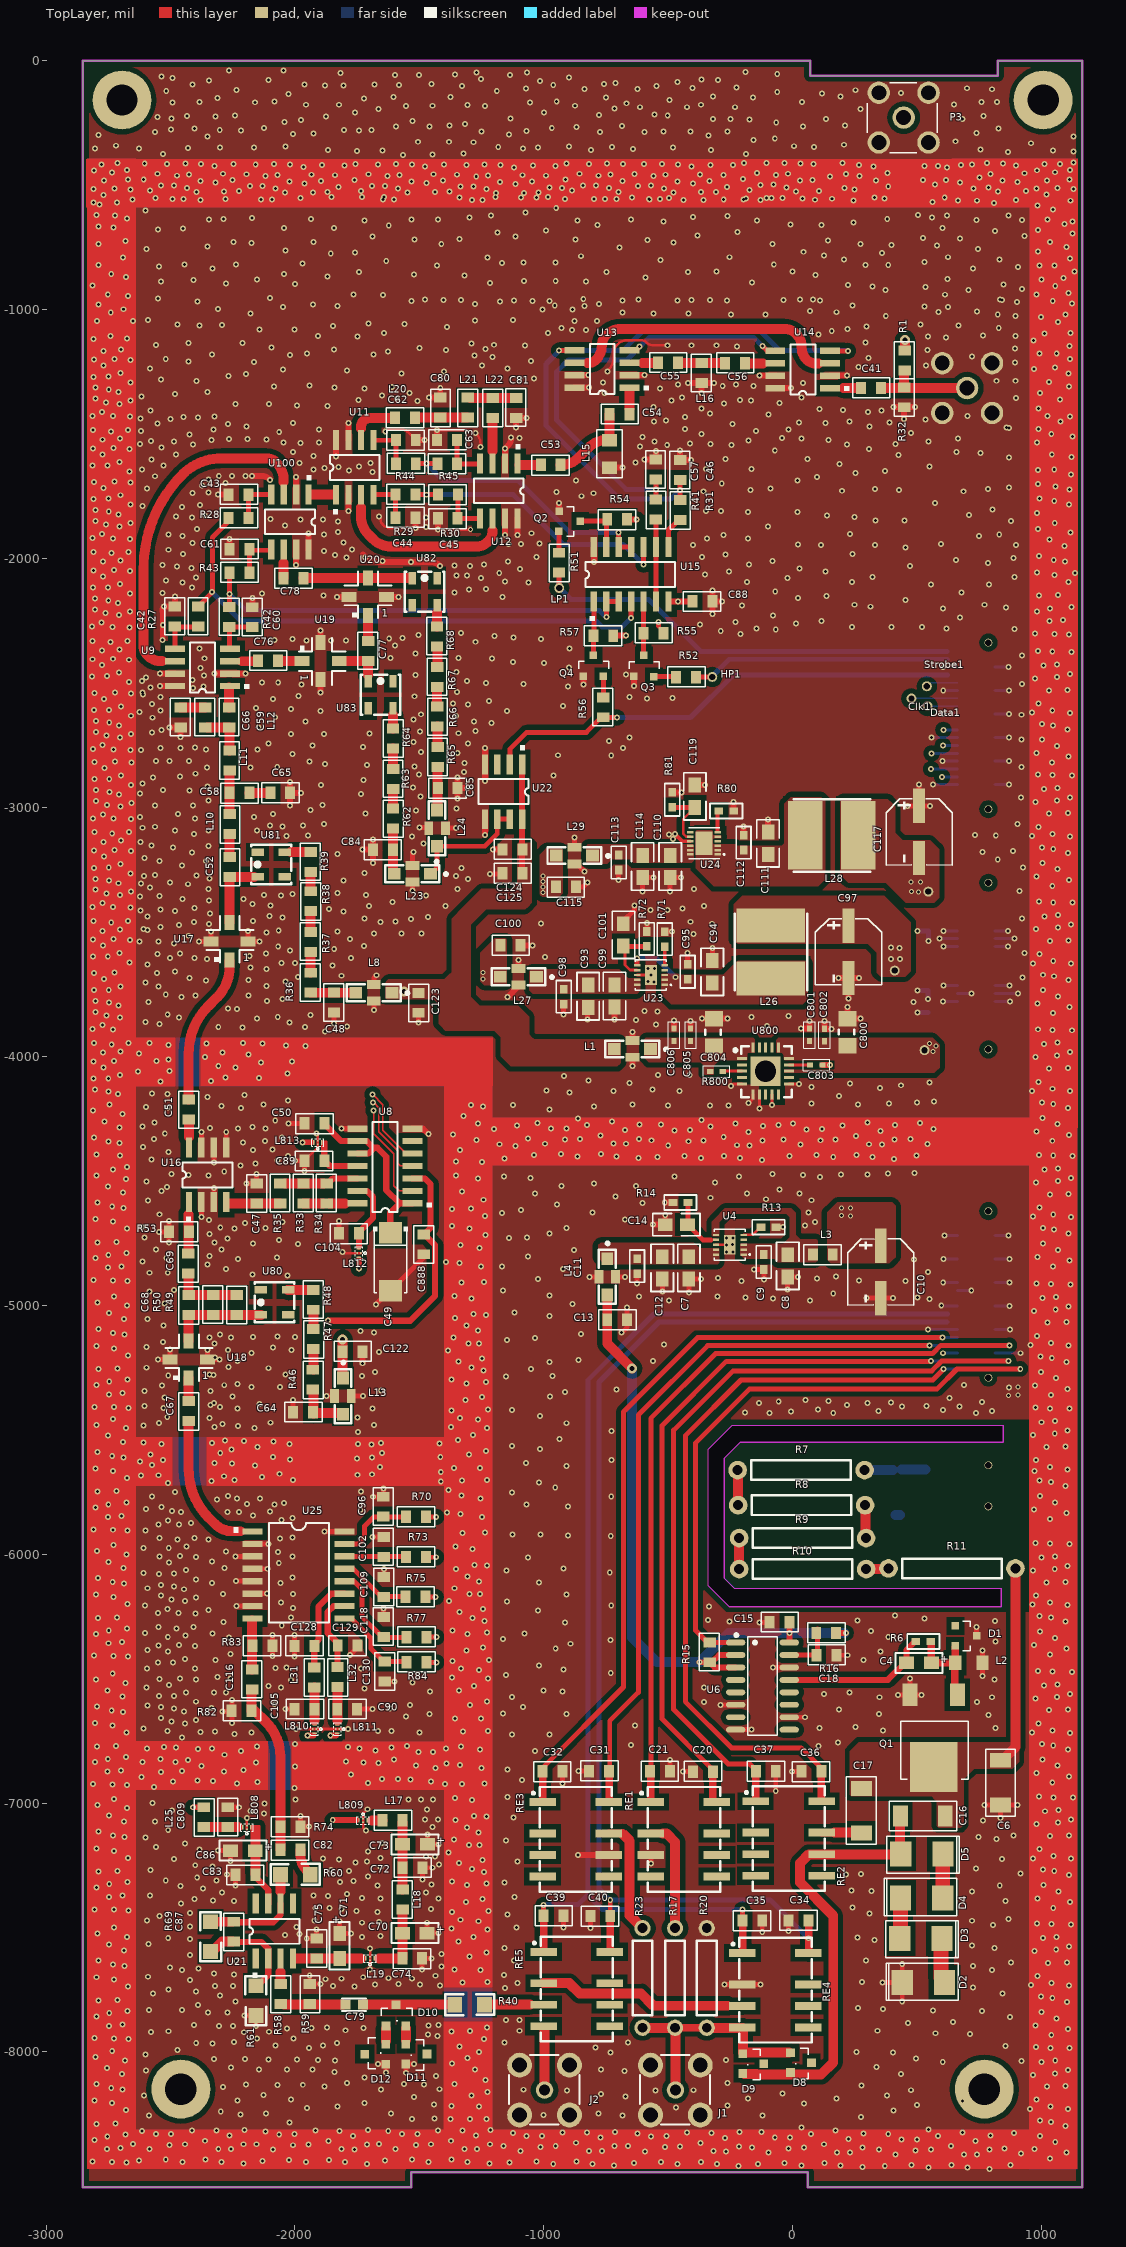
[diagram p0: TopLayer view]
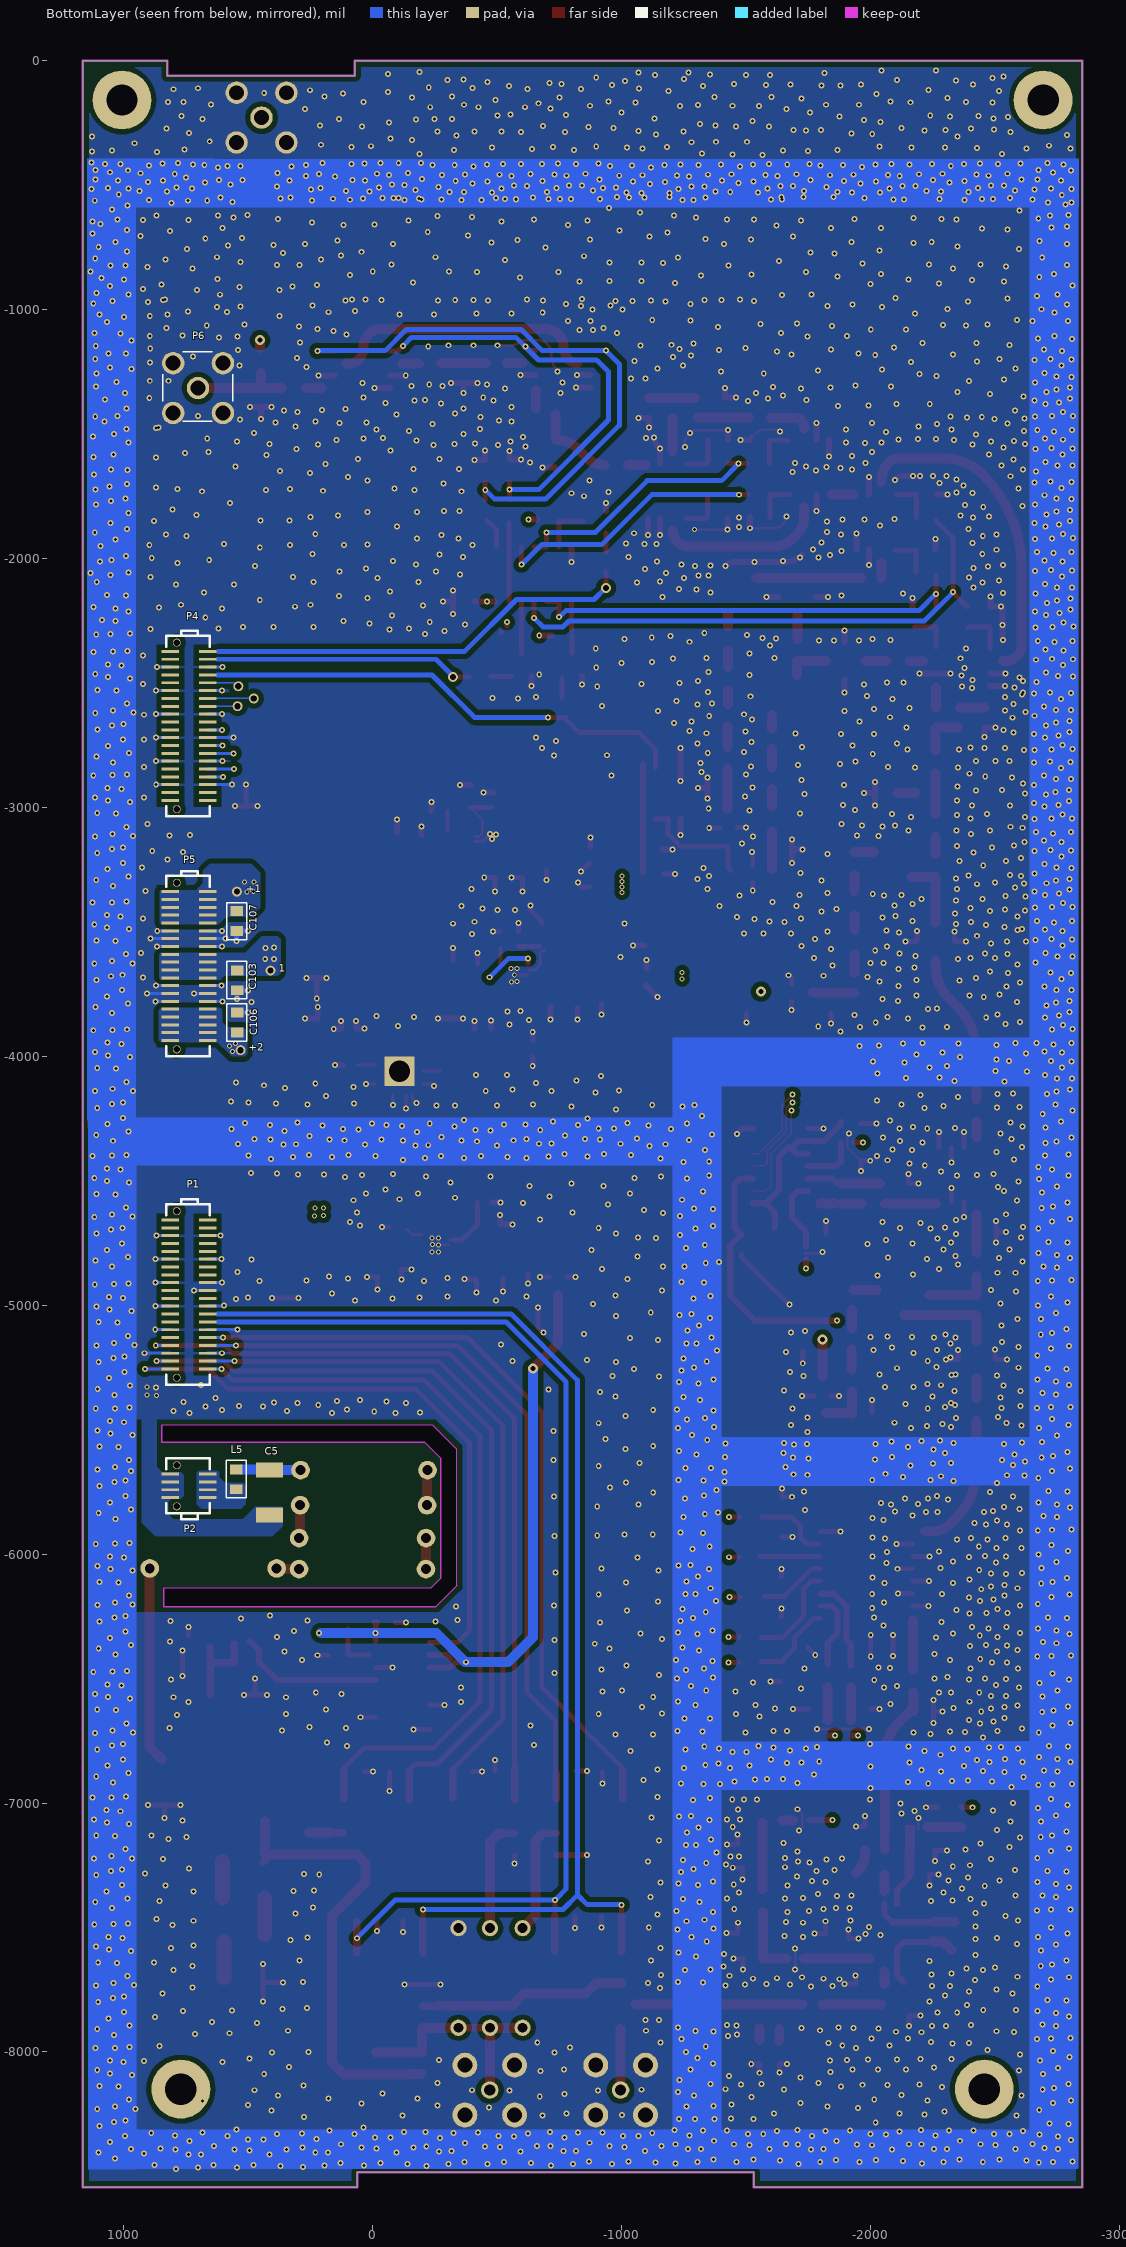
[diagram p1: BottomLayer view, seen from below]
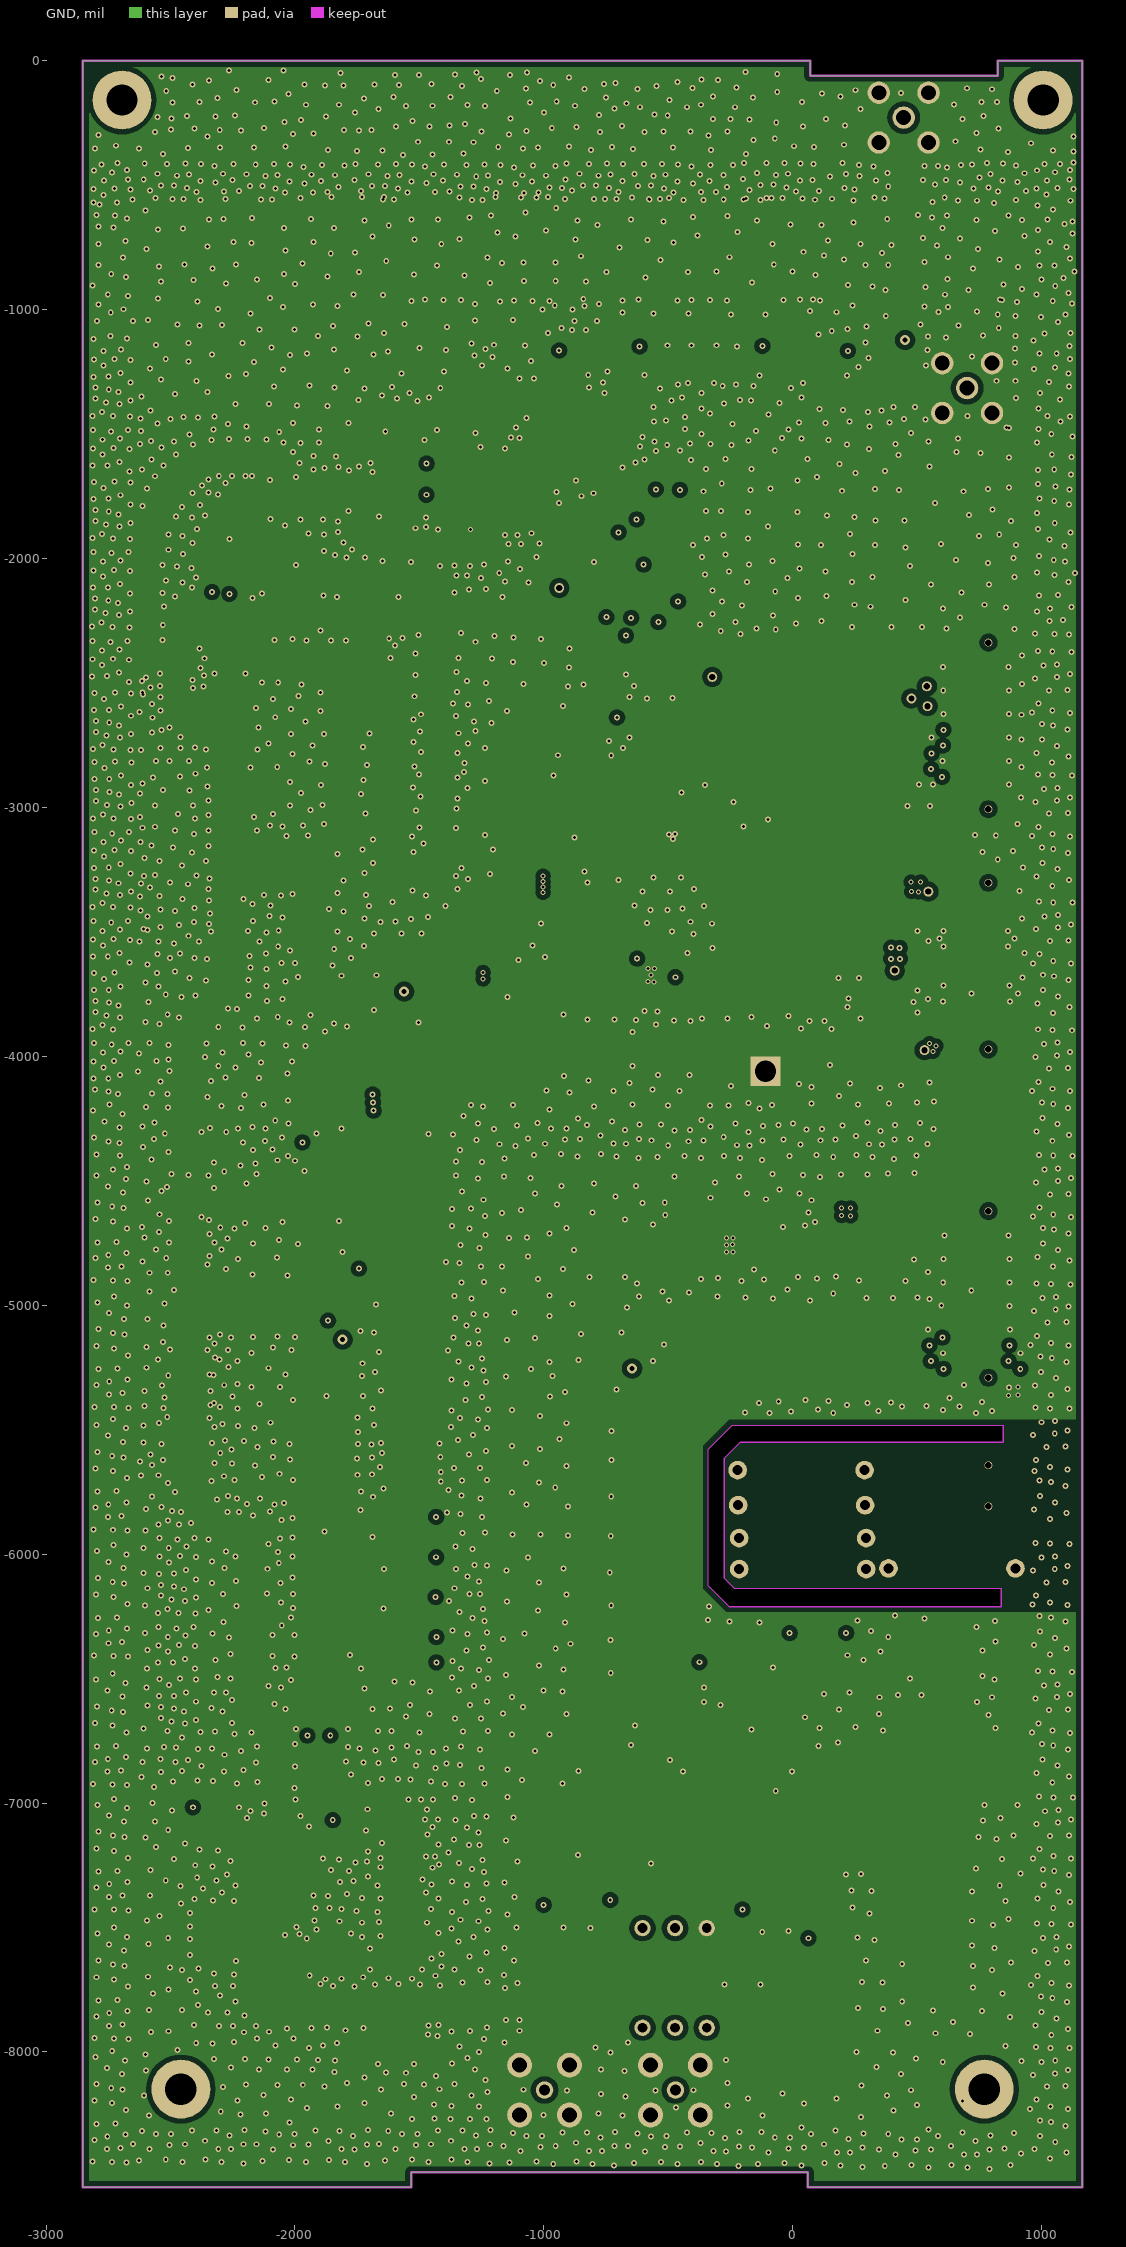
[diagram p2: GND]
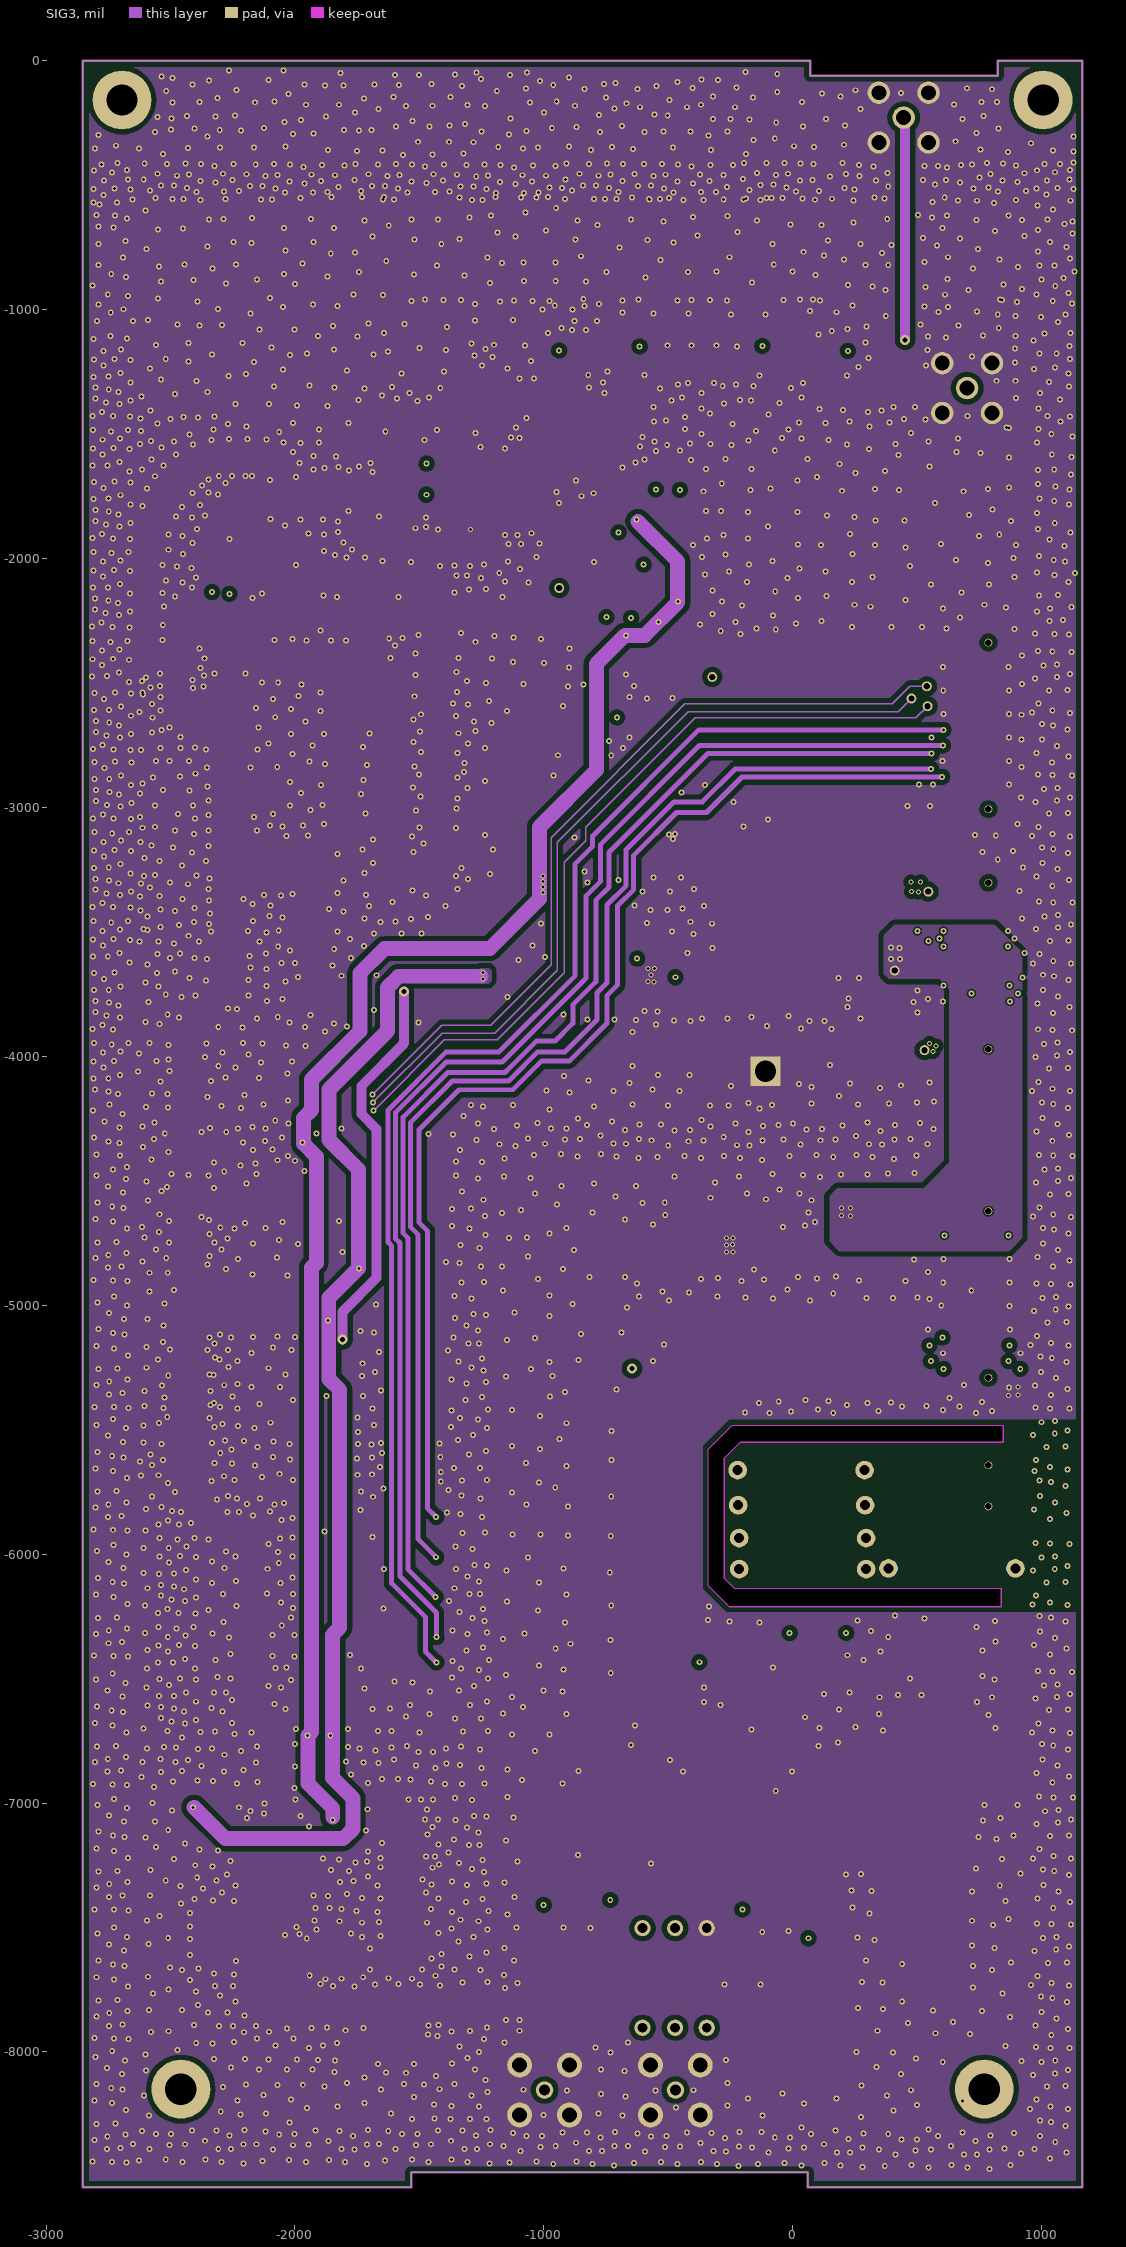
[diagram p3: SIG3]
# Altium PCB MISC109560.PcbDoc (part 1 of 7)
Units mil, origin at the board's own origin, x right, y up, seen from the top; angles counter-clockwise.
Board outline 4015.75 x 8543.31 mil, 4 copper layers (TopLayer, GND, SIG3, BottomLayer); 280 components, 173 nets, 936 pads, 3695 vias.

## Layer stack, top to bottom (the 12.6 mil dielectric is the usual default, probably not edited)
TopLayer: signal copper 1.4
Dielectric: core 12.6, FR-4, Dk 4.8
GND: signal copper 1.4
Dielectric: prepreg 12.6, FR-4, Dk 4.8
SIG3: signal copper 1.4
Dielectric: core 12.6, FR-4, Dk 4.8
BottomLayer: signal copper 1.4

## Board outline
-2852,-8543.31 -2852,0 70.78,0 70.78,-59.06 824.22,-59.06 824.22,0 1163.75,0 1163.75,-8543.31 60.7,-8543.31 60.7,-8484.25 -1532.7,-8484.25 -1532.7,-8543.31
cut-out: -339,-6127.31 -339,-5578.31 -242,-5481.31 847,-5481.31 847,-5551.31 -210,-5551.31 -274,-5615.31 -274,-6096.31 -234,-6136.31 838,-6136.31 838,-6211.31 -255,-6211.31

## Design rules (kind name [scope] priority, off if disabled: settings)
Clearance Clearance_2 [inpolygon] p1: gap=6
Clearance Clearance_1 [(IsKeepOut)] p2 off: gap=1
Clearance [All] p3: gap=6
ComponentClearance [All] p1 off: gap=10 collisioncheckmode=3 verticalgap=10 showdistances=FALSE
DiffPairsRouting [All] p1: maxlimit=6 minlimit=6 mostfreqgap=6 maxuncoupledlength=500
FabricationTestPointUsage TestPointUsage [All] p1: valid=0 allowmultiple=FALSE
FabricationTestpoint Testpoint [All] p1: side=3 testpointundercomponent=TRUE minsize=40 maxsize=100 preferedsize=60 minholesize=20 maxholesize=40 preferedholesize=32 testpointgrid=1 allowsidetop=TRUE allowsidebottom=TRUE usegrid=TRUE gridtolerance=0.01
HoleSize [All] p1 off: absolutevalues=TRUE maxlimit=500 minlimit=1 maxpercent=80.000 minpercent=20.000
HoleToHoleClearance [All] p1: gap=0 allowstackedmicrovias=TRUE
MinimumSolderMaskSliver [All] p1: minsoldermaskwidth=0
PlaneClearance [All] p1: clearance=6
PlaneConnect [All] p1: planeconnectstyle=Direct reliefexpansion=20 reliefentries=4 reliefconductorwidth=10 reliefairgap=10
PolygonConnect [All] p1: connectstyle=Direct reliefconductorwidth=10 reliefentries=4 polygonreliefangle="90 Angle"
RoutingLayers [All] p1: top layer_v5=TRUE mid layer 1_v5=FALSE mid layer 2_v5=FALSE bottom layer_v5=TRUE
RoutingVias [All] p1: holewidth=12 width=20 viastyle="Through Hole" minholewidth=12 minwidth=20 maxholewidth=20 maxwidth=40
SilkToSilkClearance [All] p1: silktosilkclearance=0
SilkscreenOverComponentPads [IsPad] p1: minsilkscreentomaskgap=0
SolderMaskExpansion [All] p1: expansion=4
Width [All] p1: maxlimit=200 minlimit=5 preferedwidth=200 toplayer_minwidth=6 toplayer_prefwidth=10 midlayer1_minwidth=6 midlayer1_prefwidth=10 bottomlayer_minwidth=6 bottomlayer_prefwidth=10 minimp=50.000000 maximp=50.000000 favimp=50.000000
16 further rules are at their usual default settings.

## Components (designator, comment, footprint, x,y, rotation, side; value= is the part's Value field where it differs from the comment)
1 "" DIP-1 410,-3655.31 r270 bottom
+1 "" DIP-1 545,-3338 r0 bottom
+2 "" DIP-1 530,-3975 r0 bottom
C4 "20PF 10%" 0805C-2 557,-6437 r180 top
C5 "330PF 10%" 1812C 414,-5842.31 r90 bottom
C6 "22PF 10%" 1812C-2 835,-6828 r270 top
C7 "22uF/16V" 0805 -417,-4895 r90 top
C8 "22uF/16V" 0805 -20,-4887 r90 top
C9 "100NF 10%" 0603 -116,-4796 r270 top
C10 "220UF 25V (D6.3*7.7mm)" CAP-SMD_BD6.3-L6.6-W6.6-FD 354,-4761 r270 top
C11 "100NF 10%" 0603 -625,-4813 r270 top
C12 "22uF/16V" 0805 -524,-4895 r90 top
C13 "100NF 10%" 0805R -745,-5059 r0 top
C14 "22uF  16V" 0805 -422,-4676 r180 top
C15 "100NF 10%" 0805R -93,-6273.69 r0 top
C16 "47PF 10%" 1812C-2 433,-7052 r0 top
C17 "100PF 10%" 1812C-2 276,-7121 r90 top
C18 "20PF 10%" 0805R 95.8,-6405.81 r0 top
C20 "100NF 10%" 0805R -401,-6873.59 r0 top
C21 "100NF 10%" 0805R -493,-6871.59 r180 top
C31 "100NF 10%" 0805R -817.66,-6872 r0 top
C32 "100NF 10%" 0805R -925,-6872.59 r180 top
C34 "100NF 10%" 0805R -17.26,-7472 r0 top
C35 "100NF 10%" 0805R -122.26,-7472 r180 top
C36 "100NF 10%" 0805R 115,-6872.59 r180 top
C37 "100NF 10%" 0805R -148,-6872.59 r0 top
C39 "100NF 10%" 0805R -1001,-7453.59 r0 top
C40 "100NF 10%" 0805R -732.96,-7454 r180 top
C41 "100NF 10%" 0805R 275,-1314.31 r0 top
C42 "100NF 10%" 0805R -2482.59,-2272.27 r90 top
C43 "100NF 10%" 0805R -2265.96,-1742.72 r0 top
C44 "100NF 10%" 0805R -1596.41,-1835.35 r0 top
C45 "100NF 10%" 0805R -1346,-1838.31 r180 top
C46 "100NF 10%" 0805R -452,-1684.31 r90 top
C47 "100NF 10%" 0805R -2153.96,-4510.31 r270 top
C48 "100NF 10%" 0805R -1843,-3824 r90 top
C49 "22uF 25V" CAP-SMD_L6.0-W3.2-R-RD -1616,-4708 r90 top
C50 "100NF 10%" 0805R -1880.96,-4269.31 r180 top
C51 "100NF 10%" 0805R -2426.96,-4173.31 r270 top
C52 "100NF 10%" 0805R -2262,-3199 r270 top
C53 "3.3NF 10%" 0805R -932,-1623 r180 top
C54 "100NF 10%" 0805R -736,-1420 r0 top
C55 "330PF 10%" 0805R -540.96,-1213.09 r0 top
C56 "330PF 10%" 0805R -272,-1214.68 r0 top
C57 "100NF 10%" 0805R -550,-1682.31 r90 top
C58 "33PF 10%" 0805R -2182,-2941.31 r180 top
C59 "33PF 10%" 0805R -2360.96,-2677.72 r90 top
C60 "100NF 10%" 0805R -2170.59,-2275.27 r90 top
C61 "100NF 10%" 0805R -2263,-1962.31 r0 top
C62 "100NF 10%" 0805R -1514.41,-1523.35 r180 top
C63 "100NF 10%" 0805R -1428.41,-1523.35 r0 top
C64 "100NF 10%" 0805R -2007,-5429.96 r0 top
C65 "33PF 10%" 0805R -2099,-2941.31 r0 top
C66 "33PF 10%" 0805R -2458.96,-2677.72 r90 top
C67 "100NF 10%" 0805R -2426.96,-5385.31 r270 top
C68 "39PF 10%" 0805R -2426.96,-4959.31 r270 top
C69 "100NF 10%" 0805R -2428.96,-4792.31 r270 top
C70 "25V 1UF Type A" 0805C-2 -1468.48,-7523 r180 top
C71 "25V 1UF Type A" 0805C-2 -1820.48,-7524 r270 top
C72 "100NF 10%" 0805R -1567.48,-7260 r0 top
C73 "25V 1UF Type A" 0805C-2 -1467.48,-7166 r180 top
C74 "100NF 10%" 0805R -1488.48,-7624 r180 top
C75 "100NF 10%" 0805R -1912.48,-7544 r270 top
C76 "10NF 10%" 0805R -2148,-2410.31 r0 top
C77 "10NF 10%" 0805R -1706,-2411.31 r90 top
C78 "10NF 10%" 0805R -1965,-2078.31 r180 top
C79 "100NF 10%" 0603C -1727,-7810 r180 top
C80 "33PF 10%" 0805R -1416,-1353.31 r270 top
C81 "33PF 10%" 0805R -1111,-1434.31 r90 top
C82 "100NF 10%" 0805R -1978.48,-7188 r180 top
C83 "100NF 10%" 0805R -2158.48,-7288 r180 top
C84 "100NF 10%" 0805R -1606,-3169.31 r180 top
C85 "100NF 10%" 0805R -1346,-2921.61 r180 top
C86 "25V 1UF Type A" 0805C-2 -2159.26,-7191.41 r180 top
C87 "3pF( ±0.1pF)" 0805R -2246.48,-7477 r270 top
C88 "100NF 10%" 0805R -323,-2171.31 r180 top
C89 "100NF 10%" 0805R -1881.96,-4419.31 r180 top
C90 "100NF 10%" 0805R -1829.93,-6623.01 r0 top
C93 "22uF/16V" 0805 -822,-3803.31 r90 top
C94 "22uF/16V" 0805 -323,-3615 r270 top
C95 "100NF 10%" 0603 -422,-3690 r90 top
C96 "100NF 10%" 0805R -1644.89,-5849.42 r90 top
C97 "220UF 25V (D6.3*7.7mm)" CAP-SMD_BD6.3-L6.6-W6.6-FD 224,-3475 r270 top
C98 "100NF 10%" 0603 -920,-3730 r270 top
C99 "22uF/16V" 0805 -716,-3802.31 r90 top
C100 "100NF 10%" 0805R -1174,-3554 r0 top
C101 "22uF  16V" 0805 -680,-3557 r90 top
C102 "100NF 10%" 0805R -1643.89,-6011.42 r90 top
C103 "100NF 10%" 0805R 544,-3734.31 r90 bottom
C104 "100NF 10%" 0805R -1742.96,-4711.31 r180 top
C105 "100NF 10%" 0805R -2000.93,-6623.01 r0 top
C106 "100NF 10%" 0805R 544,-3904.31 r90 bottom
C107 "100NF 10%" 0805R 546,-3416.31 r270 bottom
C109 "100NF 10%" 0805R -1642.89,-6172.42 r90 top
C110 "22uF/16V" 0805 -492,-3282 r90 top
C111 "22uF/16V" 0805 -99,-3099 r270 top
C112 "100NF 10%" 0603 -197,-3171 r90 top
C113 "100NF 10%" 0603 -699,-3191 r270 top
C114 "22uF/16V" 0805 -603,-3282 r90 top
C115 "100NF 10%" 0805R -871,-3319 r180 top
C116 "100NF 10%" 0805R -2171.71,-6543.69 r90 top
C117 "220UF 25V (D6.3*7.7mm)" CAP-SMD_BD6.3-L6.6-W6.6-FD 508,-2993 r270 top
C118 "100NF 10%" 0805R -1643.93,-6332.01 r90 top
C119 "22uF  16V" 0805 -393,-3000 r90 top
C122 "100NF 10%" 0805R -1808.73,-5186 r0 top
C123 "100NF 10%" 0805R -1503.43,-3744.61 r270 top
C124 "100NF 10%" 0805R -1166,-3168.69 r0 top
C125 "100NF 10%" 0805R -1166,-3264.69 r0 top
C128 "100NF 10%" 0805R -2001.93,-6369.01 r0 top
C129 "100NF 10%" 0805R -1747.93,-6367.01 r180 top
C130 "100NF 10%" 0805R -1639.93,-6431.01 r270 top
C800 "47uF 25V" 1206 220,-3958 r180 top
C801 "0.1uF" 0402 67,-3938.31 r90 top
C802 "1uF 25V" 0402 127,-3939.31 r90 top
C803 "1uF 25V" 0402 70,-4034 r0 top
C804 "47uF 25V" 1206 -316,-3958.31 r180 top
C805 "0.1uF" 0402 -410,-3938.31 r90 top
C806 "1uF 25V" 0402 -477,-3938.31 r90 top
C809 "100nF 10%" 0805R -2269,-7097 r90 top
C888 "100nF 10%" 0805R -1483,-4715 r270 top
Clk1 "" DIP-1 477,-2562 r270 top
D1 "BAV99/A7" SOT-23 654,-6288 r270 top
D2 "GF1M-E3/67A/GM" 1808D 610.22,-7720.99 r180 top
D3 "GF1M-E3/67A/GM" 1808D 430,-7544 r0 top
D4 "GF1M-E3/67A/GM" 1808D 603,-7381 r180 top
D5 "GF1M-E3/67A/GM" 1808D 434,-7205 r0 top
D8 "BAV99/A7" SOT-23-2 -9,-8003 r270 top
D9 "BAV99/A7" SOT-23-2 -201,-8007 r270 top
D10 "BAV99/A7" SOT-23-2 -1634.26,-7895.69 r0 top
D11 "BAV99/A7" SOT-23-2 -1554.26,-7968.69 r270 top
D12 "BAV99/A7" SOT-23-2 -1634.48,-8049 r90 top
Data1 "" DIP-1 542,-2593 r270 top
HP1 "" DIP-1 -323,-2475.31 r270 top
J1 "RF connector" DIP-P -571.26,-8253.31 r90 top locked
J2 "RF connector" DIP-P -1097,-8253.31 r90 top locked
L1 "YFF31HC2A105MT000N" FILTER-SMD_4P-L3.2-W1.6-L_YFF31HC -571,-3970 r180 top
L2 "15UH 5%" 1005R 652.78,-6436.31 r0 top
L3 "BLM21PG221SN1D(220Ω@100MHz)" 0805R 161,-4796 r180 top
L4 "YFF31HC2A105MT000N" FILTER-SMD_4P-L3.2-W1.6-L_YFF31HC -745,-4813 r270 top
L5 "6.8UH 10%" 0805R 547,-5739.31 r90 bottom
L8 "YFF31HC2A105MT000N" FILTER-SMD_4P-L3.2-W1.6-L_YFF31HC -1610,-3744 r180 top
L10 "10NH 10%" 0805R -2261.96,-3026.72 r270 top
L11 "10NH 10%" 0805R -2261.96,-2851.72 r90 top
L12 "10NH 10%" 0805R -2263.96,-2677.72 r90 top
L13 "YFF31HC2A105MT000N" FILTER-SMD_4P-L3.2-W1.6-L_YFF31HC -1807,-5292 r270 top
L15 "4.7UH 5%" 1005L -736,-1524 r270 top
L16 "1UH 5%" 0805R -366,-1294.68 r90 top
L17 "BLM21PG221SN1D(220Ω@100MHz)" 0805R -1647.48,-7070 r0 top
L18 "BLM21PG221SN1D(220Ω@100MHz" 0805R -1567.48,-7428 r90 top
L19 "NFM15PC104R1A3D" FILTER-SMD_0402-3P-L1.0-W0.5-T -1698,-7615 r180 top
L20 "10NH 10%" 0805R -1598.41,-1434.35 r0 top
L21 "10NH 10%" 0805R -1306.41,-1353.35 r270 top
L22 "10NH 10%" 0805R -1205.41,-1354.35 r270 top
L23 "YFF31HC2A105MT000N" FILTER-SMD_4P-L3.2-W1.6-L_YFF31HC -1455,-3266 r180 top
L24 "YFF31HC2A105MT000N" FILTER-SMD_4P-L3.2-W1.6-L_YFF31HC -1429,-3155.61 r90 top
L25 "BLM21PG221SN1D(220Ω@100MHz" 0805R -2366,-7017 r270 top
L26 "CD75-470M(47uH/1A)" IND-SMD_L7.8-W7.0-A -88,-3687 r90 top
L27 "YFF31HC2A105MT000N" FILTER-SMD_4P-L3.2-W1.6-L_YFF31HC -1029,-3680 r180 top
L28 "CD75-470M(47uH/1A)" IND-SMD_L7.8-W7.0-A 51,-3112 r0 top
L29 "YFF31HC2A105MT000N" FILTER-SMD_4P-L3.2-W1.6-L_YFF31HC -804,-3193 r180 top
L31 "BLM21PG221SN1D(220Ω@100MHz" 0805R -1921.93,-6536.01 r90 top
L32 "BLM21PG221SN1D(220Ω@100MHz" 0805R -1828.93,-6454.01 r270 top
L808 "NFM15PC104R1A3D" FILTER-SMD_0402-3P-L1.0-W0.5-T -2193,-7089 r180 top
L809 "NFM15PC104R1A3D" FILTER-SMD_0402-3P-L1.0-W0.5-T -1726,-7079 r0 top
L810 "NFM15PC104R1A3D" FILTER-SMD_0402-3P-L1.0-W0.5-T -1930,-6703 r270 top
L811 "NFM15PC104R1A3D" FILTER-SMD_0402-3P-L1.0-W0.5-T -1838,-6703 r270 top
L812 "NFM15PC104R1A3D" FILTER-SMD_0402-3P-L1.0-W0.5-T -1751.96,-4790.31 r270 top
L813 "NFM15PC104R1A3D" FILTER-SMD_0402-3P-L1.0-W0.5-T -1908,-4337 r180 top
LP1 "" DIP-1 -938,-2118 r180 top
P1 "Header 20X2" N0.8mm/40Pin-Plug 812.04,-4657.31 r270 bottom locked
P2 "Header 4X2" N0.8mm/8Pin-SOCKET 812.04,-5772.72 r270 bottom locked
P3 "RF connector SMB-JWHD SMB right-angle male plug, extended" DIP-P-2 346,-328 r90 top locked (schematic designator P10)
P4 "Header 20X2" N0.8mm/40Pin-Plug 812.04,-2372.83 r270 bottom locked
P5 "Header 20X2" N0.8mm/40Pin-Plug 812.04,-3337.94 r270 bottom locked
P6 "RF connector SMB-JWHD SMB right-angle male plug, extended" DIP-P-2 801,-1214.68 r180 bottom locked
Q1 "MJD31C" SOT-252-2 662,-6565 r180 top
Q2 "MMBT3906/2A" SOT-23 -938.59,-1809.27 r270 top
Q3 "MMBT3906/2A" SOT-23 -638,-2473.31 r0 top
Q4 "MMBT3906/2A" SOT-23 -841,-2472.31 r0 top
R1 "0R" 0805R 450,-1244 r90 top
R6 "2K 5%" 0603 555,-6351 r180 top
R7 "NC" AXIAL-0.51 34,-5662.31 r180 top
R8 "3.9K 5% 1/2W" AXIAL-0.51 36,-5803.31 r180 top
R9 "3.9K 5% 1/2W" AXIAL-0.51 40,-5935.31 r180 top
R10 "3.9K 5% 1/2W" AXIAL-0.51 40.22,-6059.94 r180 top
R11 "3.9K 5% 1/2W" AXIAL-0.51 640,-6057.31 r0 top
R13 "0R1%" 0603 -127,-4686 r0 top
R14 "49.9K 1%" 0603 -421,-4587 r180 top
R15 "4.99K 1%" 0805R -334,-6434.31 r90 top
R16 "2K 1%" 0805R 94.8,-6316.81 r0 top
R17 "49.9R 1% 1/4W" AXIAL-0.4 -472.26,-7703 r90 top
R20 "100R 1% 1/4W" AXIAL-0.4 -345.26,-7703 r90 top
R23 "100R 1% 1/4W" AXIAL-0.4 -603.26,-7703 r90 top
R27 "4.87K 1%" 0805R -2388.59,-2272.27 r90 top
R28 "4.87K 1%" 0805R -2265.96,-1836.72 r0 top
R29 "4.87K 1%" 0805R -1596.41,-1742.21 r0 top
R30 "4.87K 1%" 0805R -1345.41,-1742.35 r180 top
R31 "4.87K 1%" 0805R -452,-1765.31 r270 top
R32 "10K 1%" 0805R 448,-1311.68 r270 top
R33 "100K 1%" 0805R -1965.41,-4590.31 r90 top
R34 "100K 1%" 0805R -1872.37,-4590.35 r90 top
R35 "49.9R 1%" 0805R -2058.96,-4590.31 r90 top
R36 "49.9R 1%" 0805R -1937.27,-3744 r90 top
R37 "49.9R 1%" 0805R -1937.27,-3580 r90 top
R38 "49.9R 1%" 0805R -1937.27,-3336.41 r270 top
R39 "49.9R 1%" 0805R -1937,-3259 r90 top
R40 "49.9R 1% 1/4W" R-SMD_L3.5-W1.5 -1238,-7810 r180 top
R41 "10K 1%" 0805R -550,-1763.31 r270 top
R42 "4.87K 1%" 0805R -2263.59,-2274.27 r90 top
R43 "4.87K 1%" 0805R -2263,-2056.31 r0 top
R44 "4.87K 1%" 0805R -1594.41,-1618.35 r0 top
R45 "4.87K 1%" 0805R -1348,-1618.31 r180 top
R46 "169R 1%" 0805R -1928,-5259 r270 top
R47 "169R 1%" 0805R -1926,-5096 r270 top
R48 "169R 1%" 0805R -1926,-5018 r90 top
R49 "49.9R 1%" 0805R -2232.96,-5039.31 r90 top
R50 "49.9R 1%" 0805R -2328.96,-5038.31 r90 top
R51 "10K 1%" 0805R -939,-1976.31 r270 top
R52 "10K 1%" 0805R -468,-2476.31 r0 top
R53 "10K 1%" 0805R -2505.96,-4705.31 r0 top
R54 "10K 1%" 0805R -665,-1842.31 r180 top
R55 "10K 1%" 0805R -599,-2299.31 r0 top
R56 "10K 1%" 0805R -762,-2637.31 r90 top
R57 "10K 1%" 0805R -721,-2309.31 r180 top
R58 "49.9R 1%" 0805R -2057.44,-7727.41 r270 top
R59 "4.99K 1%" 0805R -1940.44,-7727.41 r270 top
R60 "49.9R 1%" R-SMD_L3.5-W1.5 -2058.09,-7287.69 r0 top
R61 "30R 1%" R-SMD_L3.5-W1.5 -2156.44,-7853.41 r90 top
R62 "169R 1%" 0805R -1606,-3004.31 r270 top
R63 "169R 1%" 0805R -1605,-2925.31 r90 top
R64 "169R 1%" 0805R -1606,-2682.31 r270 top
R65 "49.9R 1%" 0805R -1426,-2837.61 r90 top
R66 "49.9R 1%" 0805R -1428,-2594.61 r270 top
R67 "49.9R 1%" 0805R -1428,-2515.61 r90 top
R68 "49.9R 1%" 0805R -1429,-2352.31 r90 top
R69 "120R 1%" R-SMD_L3.5-W1.5 -2339.48,-7477 r270 top
R70 "169R 1%" 0805R -1553.89,-5850.42 r0 top
R71 "0R1%" 0603 -514,-3559 r90 top
R72 "49.9K 1%" 0603 -586,-3558 r90 top
R73 "169R 1%" 0805R -1553.89,-6011.42 r0 top
R74 "NC" 0805R -1978.48,-7095 r180 top
R75 "169R 1%" 0805R -1555.89,-6171.42 r0 top
R77 "169R 1%" 0805R -1551.93,-6333.01 r0 top
R80 "0R1%" 0603 -297,-3014 r0 top
R81 "49.9K 1%" 0603 -484,-2999 r90 top
R82 "100K 1%" 0805R -2254,-6630 r0 top
R83 "10K 1%" 0805R -2090.71,-6367.69 r180 top
R84 "169R 1%" 0805R -1551.93,-6434.01 r0 top
R800 "0R" 0402 -331,-4060 r0 top
RE1 "#NAME?" RELAY-SMD_PANASONIC_AGQ2X0AXX -569.66,-6996 r270 top
RE2 "#NAME?" RELAY-SMD_PANASONIC_AGQ2X0AXX -148.66,-6993 r270 top
RE3 "#NAME?" RELAY-SMD_PANASONIC_AGQ2X0AXX -1004.66,-6996 r270 top
RE4 "#NAME?" RELAY-SMD_PANASONIC_AGQ2X0AXX -202,-7602.59 r270 top
RE5 "#NAME?" RELAY-SMD_PANASONIC_AGQ2X0AXX -1000.66,-7598 r270 top
Strobe1 "" DIP-1 539,-2513 r270 top
U4 "LT3045EDD#PBF" DFN-10_L3.0-W3.0-P0.50-BL-EP -197,-4796.31 r90 top
U6 "74HCT123D" SOIC-16_L9.9-W3.9-P1.27-LS6.0-BL -229,-6355.31 r270 top
U8 "MAX504CSD+T" SO-14 -1528.37,-4590.35 r180 top
U9 "SW-239" SO-8 -2261.59,-2512.27 r180 top
U11 "SW-239" SO-8 -1834.41,-1743.35 r90 top
U12 "SW-239" SO-8 -1106,-1618.31 r270 top
U13 "SW-239" SO-8 -655.96,-1313.09 r180 top
U14 "SW-239" SO-8 150.04,-1315.09 r180 top
U15 "74HCT04D" SO-14 -798.96,-2172.72 r90 top
U16 "AT-250(MAAV-007941)" SO-8 -2425.92,-4585.72 r90 top
U17 "MAR-3SM/A03" LCC4 -2262.96,-3612.72 r90 top
U18 "MAR-6SM/A06" LCC4 -2426.92,-5292.72 r90 top
U19 "MAR-6SM/A06" LCC4 -1972,-2411.31 r0 top
U20 "MAR-3SM/A03" LCC4 -1707,-2228.31 r90 top
U21 "MAX4106ESA+T" SO-8 -2157.44,-7624.41 r90 top
U22 "MIC4420CM" SO-8 -1086.69,-2827 r270 top
U23 "LT3045EDD#PBF" DFN-10_L3.0-W3.0-P0.50-BL-EP -514,-3712.31 r90 top
U24 "LT3094EDD#PBF" WDFN-12_L3.0-W3.0-P0.45-BL-EP -451,-3199.31 r90 top
U25 "AT65-0263" SO-16 -2170.71,-5908.69 r0 top
U80 "TCCH-80+" IND-SMD_4P-L3.8-W3.8 -2136.96,-5038.31 r90 top
U81 "TCCH-80+" IND-SMD_4P-L3.8-W3.8 -2150,-3279 r90 top
U82 "TCCH-80+" IND-SMD_4P-L3.8-W3.8 -1529,-2078 r0 top
U83 "TCCH-80+" IND-SMD_4P-L3.8-W3.8 -1706,-2492 r0 top
U100 "SW-239" SO-8 -1944.96,-1742.72 r270 top
U800 "TPS7A4701RGWR" QFN-20 -203,-4008.31 r0 top

## Footprints (in the part's own frame and the unit in brackets; to place one, negate y for a bottom-side part, rotate by r counter-clockwise, add the part's x,y. Pads: shape width x height; smd on the part's side, far side on the other; paste and mask are expansions set on the pad)
0402 [mil]
  rect 25x20 smd: 1(0,0) 2(50,0)
  silkscreen extent -28,-23 78,22
0603 [mil]
  rect 35x30 smd: 1(0,0) 2(60,0)
  silkscreen extent -35,-30 95,30
0603C [mil]
  rect 40x40 smd: 1(0,0) 2(70,0)
  silkscreen extent -13,-25 83,25
0805 [mil]
  rect 60x50 smd: 1(0,0) 2(90,0)
  silkscreen extent -50,-45 140,45
0805C-2 [mil]
  rect 60x50 smd: 1(0,0) 2(100,0)
  silkscreen extent -45,-40 144,40
0805R [mil]
  rect 40x50 smd: 1(0,0) 2(80,0)
  silkscreen extent -34,-39 116,41
1005L [mil]
  rect 50x60 smd: 1(0,0) 2(110,0)
  silkscreen extent -41,-51 152,52
1005R [mil]
  rect 50x60 smd: 1(0,0) 2(110,0)
1206 [mil]
  rect 72x62 smd: 1(0,0) 2(0,-110)
  silkscreen extent -27,-65 36,-46
1808D [mil]
  rect 85x100 smd: 1(0,0) 2(170,0)
  silkscreen extent -56,-78 235,72
1812C [mil]
  rect 60x110 smd: 1(0,0) 2(180,0)
1812C-2 [mil]
  rect 60x85 smd: 1(0,0) 2(180,0)
  silkscreen extent -44,-60 226,60
AXIAL-0.4 [mil]
  round 65 hole 40: 1(-200,0) 2(200,0)
  silkscreen extent -150,-39 150,39
AXIAL-0.51 [mil]
  round 75 hole 40: 1(255,0) 2(-255,0)
  silkscreen extent -200,-40 200,39
CAP-SMD_BD6.3-L6.6-W6.6-FD [mm]
  rect 3.5x1.2 smd: 1(0,0) 2(5.34,0)
  silkscreen extent -0.71,-3.38 6.05,3.38
CAP-SMD_L6.0-W3.2-R-RD [mil]
  rect 86.91x93.54 smd: 1(0,0) 2(-233.16,0)
  silkscreen extent -242,-69 23,69
DFN-10_L3.0-W3.0-P0.50-BL-EP [mm]
  rect 0.25x0.65 smd: 1(0,0) 2(0.5,0) 3(1,0) 4(1.5,0) 5(2,0) 6(2,2.823) 7(1.5,2.823) 8(1,2.823) 9(0.5,2.823) 10(0,2.823)
  rect 2x1.2 smd: 11(1,1.411)
  silkscreen extent -0.58,-0.69 2.58,2.99
DIP-1 [mil]
  round 40 hole 25: 1(0,0)
DIP-P [mil]
  round 100 hole 60: 1(0,0) 2(0,-200) 3(200,-200) 4(200,0)
  round 70 hole 45: 5(100,-100)
  silkscreen extent -39,-240 240,42
DIP-P-2 [mil]
  round 90 hole 60: 1(0,0) 2(0,-200) 3(200,-200) 4(200,0) 5(100,-100)
  silkscreen extent -41,-234 240,46
FILTER-SMD_4P-L3.2-W1.6-L_YFF31HC [mm]
  rect 1.3x1.2 smd: 1(0,0) 3(3.7,0)
  rect 1.4x0.9 smd: 2(1.85,-0.85) 4(1.85,0.85)
  silkscreen extent -1.72,-0.85 4.6,0.85
FILTER-SMD_0402-3P-L1.0-W0.5-T [mm]
  rect 0.15x0.46 smd paste+0 mask+0.05: 1(-0.418,0.229) 3(0.432,0.229)
  rect 0.2x0.15 smd paste+0 mask+0.05: 2(0.007,0.404) 2(0.007,0.054)
  silkscreen extent -0.63,-0.15 0.64,0.99
IND-SMD_4P-L3.8-W3.8 [mm]
  rect 0.76x1.27 smd paste+0 mask+0.05: 1(0,0) 2(2.54,0) 3(2.54,-2.79) 4(0,-2.79)
  silkscreen extent -0.76,-3.43 3.3,0.64
IND-SMD_L7.8-W7.0-A [mm]
  rect 3.5x7 smd: 1(0,0) 2(5.4,0)
  silkscreen extent -1.2,-3.7 6.6,3.7
LCC4 [mil]
  rect 60x40 smd: 1(0,0) 3(150,0)
  rect 40x60 smd: 2(75,-75) 4(75,75)
  silkscreen extent -11,-96 176,93
N0.8mm/8Pin-SOCKET [mm]
  round 0.8 hole 0.68: 0(-3.3,0.65) 0(0.9,0.65)
  rect 0.3x1.8 smd: 1(0,0) 2(0,3.8) 3(-0.8,0) 4(-0.8,3.8) 5(-1.6,0) 6(-1.6,3.8) 7(-2.4,0) 8(-2.4,3.8)
  silkscreen extent -4,-0.4 2.2,4
N0.8mm/40Pin-Plug [mm]
  round 0.8 hole 0.68: 0(-0.9,0.65) 0(16.1,0.65)
  rect 0.3x1.8 smd: 1(0,0) 2(0,3.8) 3(0.8,0) 4(0.8,3.8) 5(1.6,0) 6(1.6,3.8) 7(2.4,0) 8(2.4,3.8) 9(3.2,0) 10(3.2,3.8) 11(4,0) 12(4,3.8) 13(4.8,0) 14(4.8,3.8) 15(5.6,0) 16(5.6,3.8) 17(6.4,0) 18(6.4,3.8) 19(7.2,0) 20(7.2,3.8) 21(8,0) 22(8,3.8) 23(8.8,0) 24(8.8,3.8) 25(9.6,0) 26(9.6,3.8) 27(10.4,0) 28(10.4,3.8) 29(11.2,0) 30(11.2,3.8) 31(12,0) 32(12,3.8) 33(12.8,0) 34(12.8,3.8) 35(13.6,0) 36(13.6,3.8) 37(14.4,0) 38(14.4,3.8) 39(15.2,0) 40(15.2,3.8)
  silkscreen extent -2.1,-0.4 16.8,4
QFN-20 [mil]
  rect 40x12 smd: 1(0,0) 2(0,-25.59) 3(0,-51.18) 4(0,-76.77) 5(0,-102.36) 11(188.98,-102.36) 12(188.98,-76.77) 13(188.98,-51.18) 14(188.98,-25.59) 15(188.98,0)
  rect 12x40 smd: 6(43.31,-145.67) 7(68.9,-145.67) 8(94.49,-145.67) 9(120.08,-145.67) 10(145.67,-145.67) 16(145.67,43.31) 17(120.08,43.31) 18(94.49,43.31) 19(68.9,43.31) 20(43.31,43.31)
  rect 120x120 hole 85: 21(94.49,-51.18)
  silkscreen extent -32,-156 198,49
R-SMD_L3.5-W1.5 [mm]
  rect 1.5x1.566 smd: 1(0,0) 2(3.035,0)
  silkscreen extent -0.98,-1.05 4.02,1.1
RELAY-SMD_PANASONIC_AGQ2X0AXX [mm]
  rect 0.8x2.7 smd paste+0 mask+0.05: 1(0,0) 2(3.2,0) 3(5.4,0) 4(7.6,0) 5(7.6,6.74) 6(5.4,6.74) 7(3.2,6.74) 8(0,6.74)
  silkscreen extent -1.53,-1.07 9.13,7.05
SO-8 [mil]
  rect 80x25 smd: 1(0,0) 2(0,-50) 3(0,-100) 4(0,-150) 5(220,-150) 6(220,-100) 7(220,-50) 8(220,0)
  silkscreen extent -79,-175 159,25
SO-14 [mil]
  rect 80x25 smd: 1(0,0) 2(0,-50) 3(0,-100) 4(0,-150) 5(0,-200) 6(0,-250) 7(0,-300) 8(220,-300) 9(220,-250) 10(220,-200) 11(220,-150) 12(220,-100) 13(220,-50) 14(220,0)
  silkscreen extent -79,-326 159,34
SO-16 [mil]
  rect 80x25 smd: 1(0,0) 2(0,-50) 3(0,-100) 4(0,-150) 5(0,-200) 6(0,-250) 7(0,-300) 8(0,-350) 9(370,-350) 10(370,-300) 11(370,-250) 12(370,-200) 13(370,-150) 14(370,-100) 15(370,-50) 16(370,0)
  silkscreen extent -76,-366 308,33
SOIC-16_L9.9-W3.9-P1.27-LS6.0-BL [mil]
  oval 23.7x77.6 smd: 1(0,0) 2(50,0) 3(100,0) 4(150,0) 5(200,0) 6(250,0) 7(300,0) 8(350,0) 9(350,215.4) 10(300,215.4) 11(250,215.4) 12(200,215.4) 13(150,215.4) 14(100,215.4) 15(50,215.4) 16(0,215.4)
  silkscreen extent -36,-3 373,168
SOT-23 [mil]
  rect 30x30 smd: 1(0,0) 2(80,-1) 3(40,85)
  silkscreen extent -18,30 101,59
SOT-23-2 [mil]
  rect 35x35 smd: 1(0,0) 2(80,0) 3(40,85)
  silkscreen extent -18,21 105,71
SOT-252-2 [mil]
  rect 60x90 smd: 1(0,0) 2(190,0)
  rect 190x200 smd: 3(95,290)
  silkscreen extent -43,107 227,339
WDFN-12_L3.0-W3.0-P0.45-BL-EP [mm]
  rect 0.252x0.665 smd: 1(0.272,-3.82) 2(0.722,-3.82) 3(1.172,-3.82) 4(1.622,-3.82) 5(2.072,-3.82) 6(2.522,-3.82) 7(2.522,-1.006) 8(2.072,-1.006) 9(1.622,-1.006) 10(1.172,-1.006) 11(0.722,-1.006) 12(0.272,-1.006)
  rect 2.4x1.7 smd: 13(1.397,-2.413)
  silkscreen extent -0.18,-4.53 2.97,-0.84